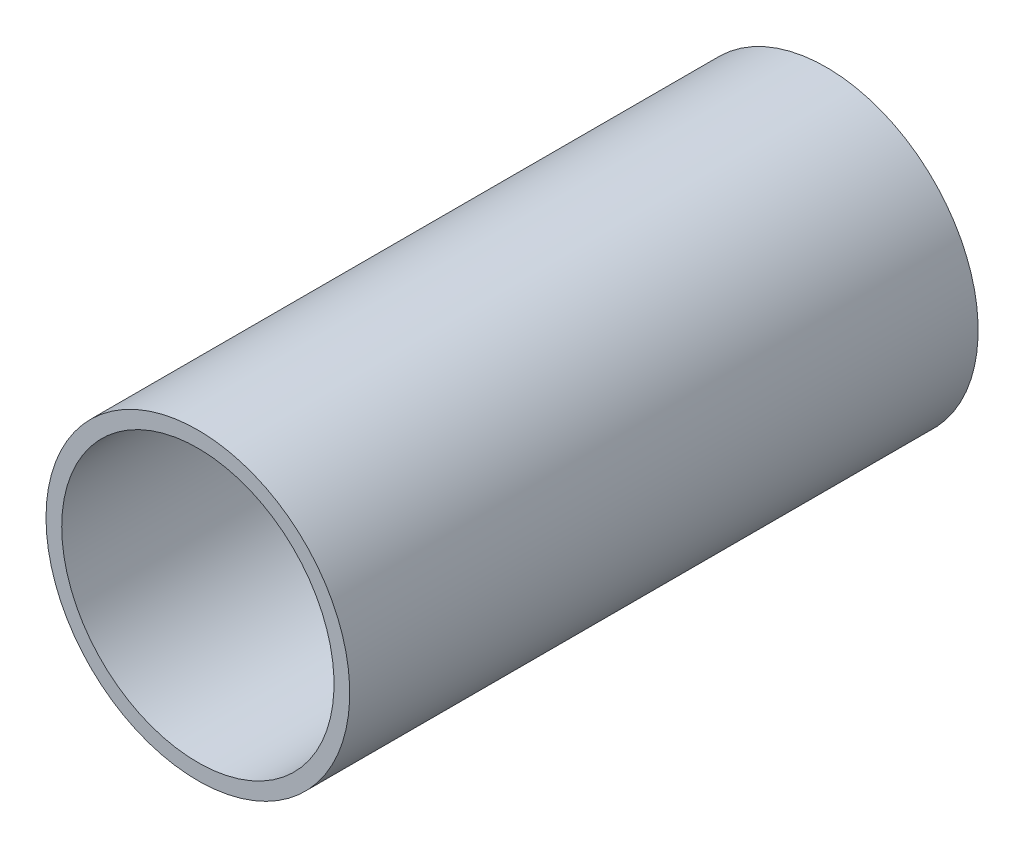
SolidWorks part; units mm, degrees
ref_plane "Front Plane" through (0, 0, 0) normal (0, 0, 1) x (1, 0, 0)
ref_plane "Top Plane" through (0, 0, 0) normal (0, 1, 0) x (1, 0, 0)
ref_plane "Right Plane" through (0, 0, 0) normal (1, 0, 0) x (0, 0, -1)
sketch "Sketch1" plane through (0, 0, 0) normal (0, 0, 1) x (1, 0, 0)
  circle A0 centre (0, 0) radius 3.683
  circle A1 centre (0, 0) radius 3.302
  dimension "D1" = 7.366
  dimension "D2" = 6.604
extrude "Boss-Extrude1" add sketch "Sketch1" along normal blind 15.24
scale "Scale1" bodies to scale 101 scale about origin uniform scaling yes scale factor 2
